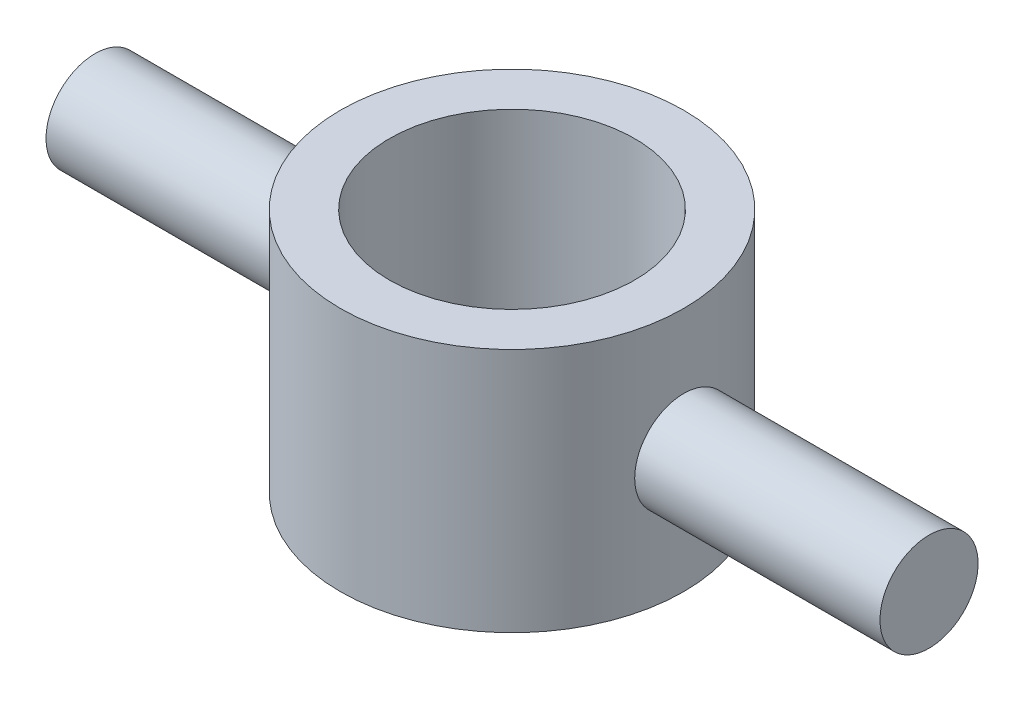
SolidWorks part; units mm, degrees
ref_plane "前视基准面" through (0, 0, 0) normal (0, 0, 1) x (1, 0, 0)
ref_plane "上视基准面" through (0, 0, 0) normal (0, 1, 0) x (1, 0, 0)
ref_plane "右视基准面" through (0, 0, 0) normal (1, 0, 0) x (0, 0, -1)
sketch "草图2" plane through (0, 0, 0) normal (0, 1, 0) x (1, 0, 0)
  circle A0 centre (0, 0) radius 7
  circle A1 centre (0, 0) radius 5
  dimension "D1" = 10
  dimension "D2" = 14
extrude "凸台-拉伸1" add sketch "草图2" along normal blind 10
ref_plane "基准面1" through (-7, 0, 0) normal (-1, 0, 0) x (0, 0, 1)
sketch "草图3" plane through (-7, 0, 0) normal (-1, 0, 0) x (0, 0, 1)
  line L0 (0, -5.5) -> (0, 5.5) construction
  line L1 (7.7, 0) -> (-7.7, 0) construction
  circle A0 centre (0, 5) radius 2
  dimension "D1" = 4
  dimension "D2" = 5
extrude "凸台-拉伸2" add sketch "草图3" along normal blind 10 separate body
mirror "镜向3" about plane through (0, 0, 0) normal (1, 0, 0) of bodies 107
